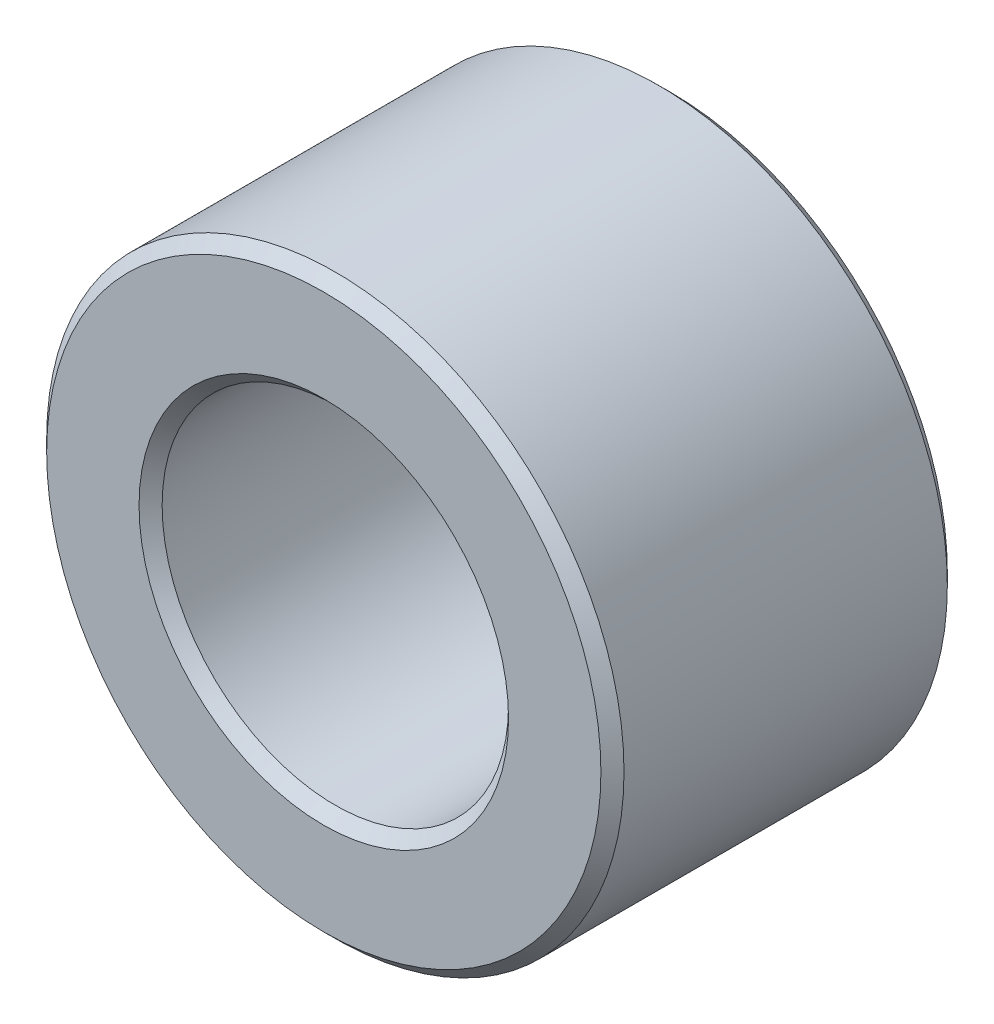
SolidWorks part; units mm, degrees
material "45#"
ref_plane "Front Plane" through (0, 0, 0) normal (0, 0, 1) x (1, 0, 0)
ref_plane "Top Plane" through (0, 0, 0) normal (0, 1, 0) x (1, 0, 0)
ref_plane "Right Plane" through (0, 0, 0) normal (1, 0, 0) x (0, 0, -1)
sketch "Sketch1" plane through (0, 0, 0) normal (0, 0, 1) x (1, 0, 0)
  circle A0 centre (0, 0) radius 25
  circle A1 centre (0, 0) radius 15
  dimension "D1" = 50
  dimension "D2" = 30
extrude "Boss-Extrude1" add sketch "Sketch1" along normal blind 30
chamfer "Chamfer1" distance 1 angle 45 4 edges at (15, 0, 0) (25, 0, 0) (15, 0, 30) (25, 0, 30)
